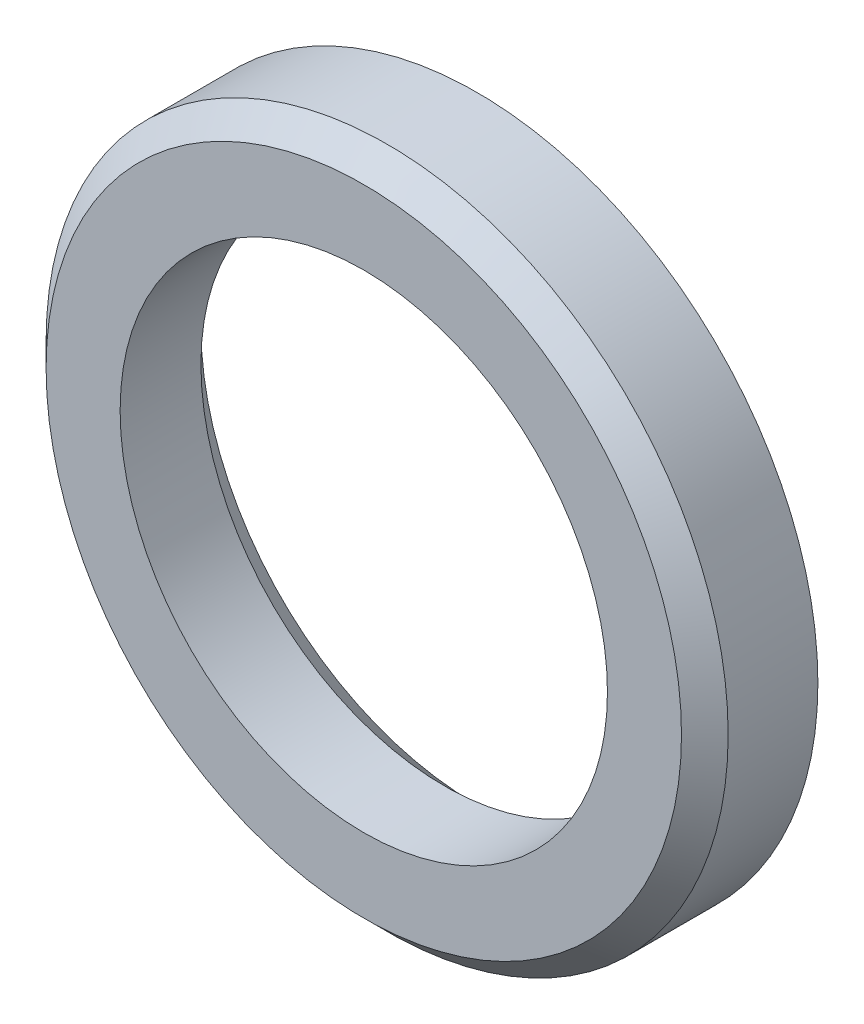
SolidWorks part; units mm, degrees
material "镀铬不锈钢"
ref_plane "前视基准面" through (0, 0, 0) normal (0, 0, 1) x (1, 0, 0)
ref_plane "上视基准面" through (0, 0, 0) normal (0, 1, 0) x (1, 0, 0)
ref_plane "右视基准面" through (0, 0, 0) normal (1, 0, 0) x (0, 0, -1)
other "Configuration Table"
sketch "草图1" plane through (0, 0, 0) normal (0, 0, 1) x (1, 0, 0)
  circle A0 centre (0, 0) radius 13.575
  circle A1 centre (0, 0) radius 19
  dimension "D1" = 27.15
  dimension "D2" = 38
extrude "凸台-拉伸1" add sketch "草图1" along normal blind 6.3
chamfer "倒角1" distance 1.3 angle 45 1 edges at (19, 0, 6.3)
chamfer "倒角2" distance 1.8 angle 45 1 edges at (13.575, 0, 0)
